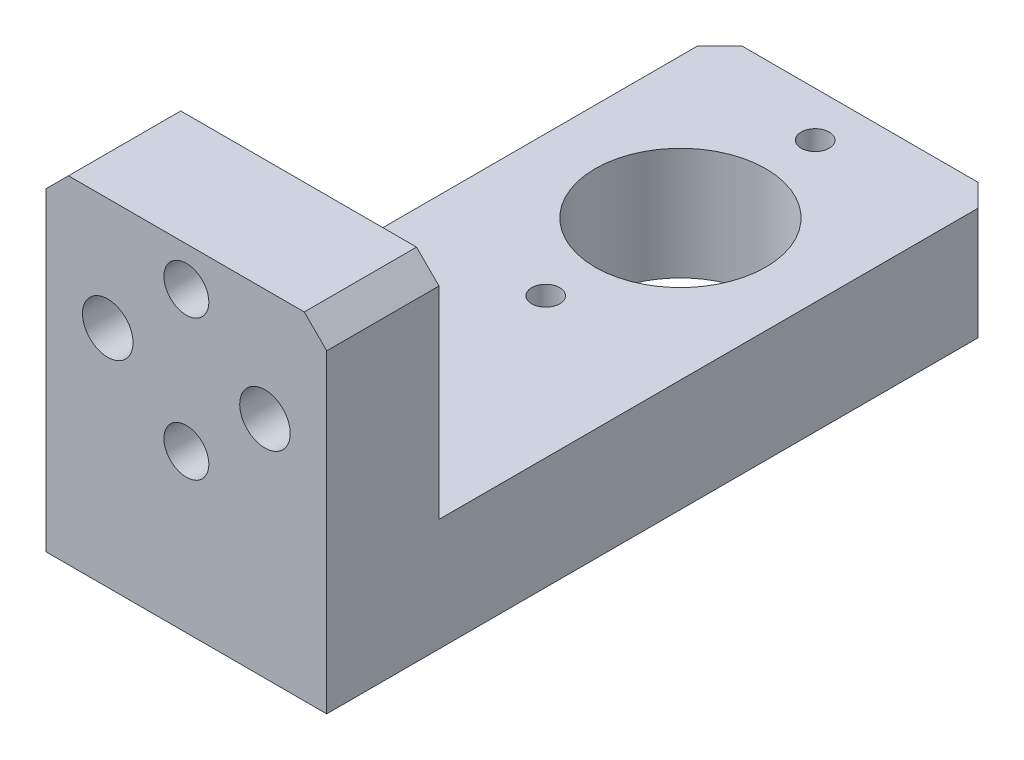
from build123d import *

# Parameters (mm, degrees)
SKETCH_1_W                = 25
SKETCH_1_H                = 60
EXTRUDE_1_DEPTH           = 10
SKETCH_2_R                = 7.6
CUT_EXTRUDE_1_DEPTH       = 20
SKETCH_3_W                = 25
SKETCH_3_H                = 10
EXTRUDE_2_DEPTH           = 20
CHAMFER_1_SIZE            = 2
HOLE_WIZARD_1_D           = 4.5
HOLE_WIZARD_1_DEPTH       = 15
HOLE_WIZARD_1_CBORE_D     = 8
HOLE_WIZARD_1_CBORE_DEPTH = 4.6
HOLE_WIZARD_1_TIP         = 1.351936393
MM_1_D                    = 4
MM_1_DEPTH                = 15
MM_1_TIP                  = 1.201721238
HOLE_WIZARD_M3_1_D        = 2.5
HOLE_WIZARD_M3_1_DEPTH    = 15
HOLE_WIZARD_M3_1_TIP      = 0.751075774


with BuildPart() as part:
    # 草图1 → 凸台-拉伸1 (new body)
    with BuildSketch(Plane(origin=(0, 0, 0), x_dir=(1, 0, 0), z_dir=(0, 1, 0))):
        Rectangle(SKETCH_1_W, SKETCH_1_H)
    extrude(amount=EXTRUDE_1_DEPTH)

    # 草图2 → 切除-拉伸1 (cut)
    with BuildSketch(Plane.XZ):
        with Locations(Location((0, -14, 0), (0, 0, 270))):
            Circle(SKETCH_2_R)
    extrude(amount=-CUT_EXTRUDE_1_DEPTH, mode=Mode.SUBTRACT)

    # 草图3 → 凸台-拉伸2 (add)
    with BuildSketch(Plane(origin=(0, 10, 0), x_dir=(1, 0, 0), z_dir=(0, 1, 0))):
        with Locations((0, -25)):
            Rectangle(SKETCH_3_W, SKETCH_3_H)
    extrude(amount=EXTRUDE_2_DEPTH)

    # 倒角1
    chamfer_1_edges = [part.edges().sort_by_distance(p)[0] for p in [
        (-12.5, 30, 25),
        (12.5, 30, 25),
        (-12.5, 5, -30),
        (12.5, 5, -30),
    ]]
    chamfer(chamfer_1_edges, length=CHAMFER_1_SIZE)

    # 打孔尺寸(%根据)内六角圆柱头螺钉的类型1
    with Locations(Plane(origin=(0, 0, 20), x_dir=(-1, 0, 0), z_dir=(0, 0, -1))):
        with Locations((7, 20), (-7, 20)):
            CounterBoreHole(HOLE_WIZARD_1_D / 2, HOLE_WIZARD_1_CBORE_D / 2, HOLE_WIZARD_1_CBORE_DEPTH, depth=HOLE_WIZARD_1_DEPTH)
            with Locations((0, 0, -(HOLE_WIZARD_1_DEPTH + HOLE_WIZARD_1_TIP / 2))):  # 118° drill point
                Cone(0, HOLE_WIZARD_1_D / 2, HOLE_WIZARD_1_TIP, mode=Mode.SUBTRACT)

    # 大小mm 暗销孔1
    with Locations(Plane(origin=(0, 0, 20), x_dir=(-1, 0, 0), z_dir=(0, 0, -1))):
        with Locations((0, 26.5), (0, 14)):
            Hole(MM_1_D / 2, depth=MM_1_DEPTH)
            with Locations((0, 0, -(MM_1_DEPTH + MM_1_TIP / 2))):  # 118° drill point
                Cone(0, MM_1_D / 2, MM_1_TIP, mode=Mode.SUBTRACT)

    # M3 螺纹孔1
    with Locations(Plane(origin=(0, 0, 0), x_dir=(-1, 0, 0), z_dir=(0, -1, 0))):
        with Locations((0, 26), (0, 2)):
            Hole(HOLE_WIZARD_M3_1_D / 2, depth=HOLE_WIZARD_M3_1_DEPTH)
            with Locations((0, 0, -(HOLE_WIZARD_M3_1_DEPTH + HOLE_WIZARD_M3_1_TIP / 2))):  # 118° drill point
                Cone(0, HOLE_WIZARD_M3_1_D / 2, HOLE_WIZARD_M3_1_TIP, mode=Mode.SUBTRACT)


solid = part.part
